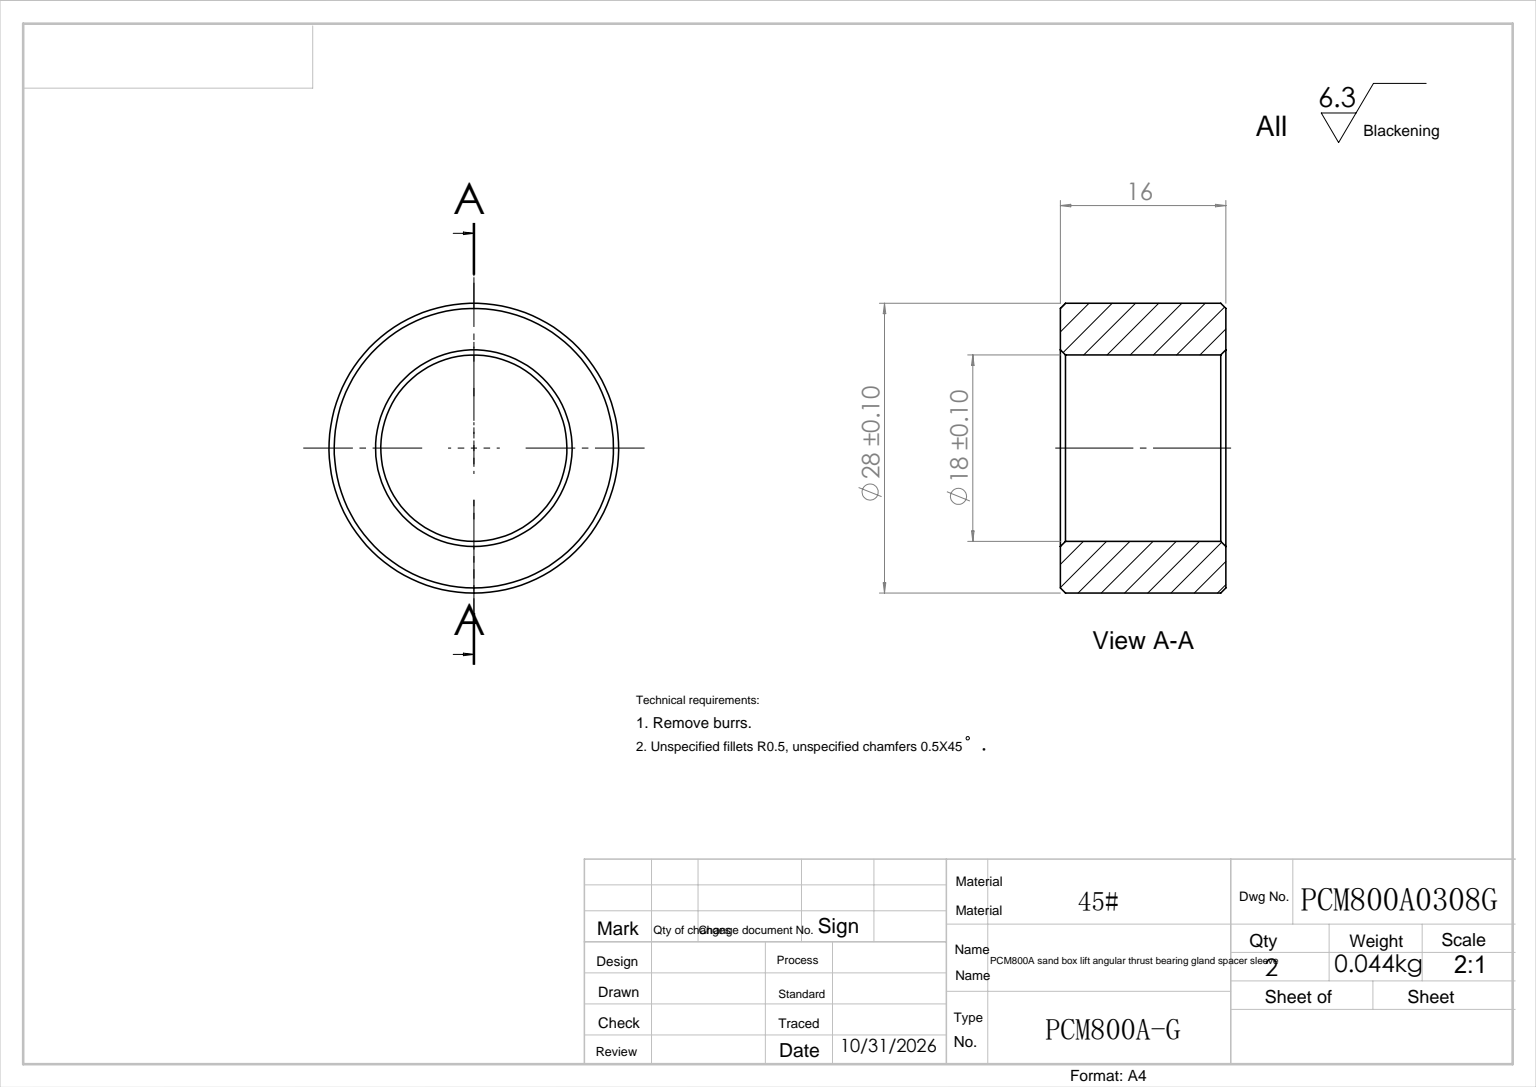
SolidWorks part; units mm, degrees
ref_plane "前视基准面" through (0, 0, 0) normal (0, 0, 1) x (1, 0, 0)
ref_plane "上视基准面" through (0, 0, 0) normal (0, 1, 0) x (1, 0, 0)
ref_plane "右视基准面" through (0, 0, 0) normal (1, 0, 0) x (0, 0, -1)
sketch "草图1" plane through (0, 0, 0) normal (0, 1, 0) x (1, 0, 0)
  circle A0 centre (0, 0) radius 14
  circle A1 centre (0, 0) radius 9
  dimension "D1" = 18
  dimension "D2" = 28
extrude "拉伸1" add sketch "草图1" along normal blind 16
chamfer "倒角1" distance 0.5 angle 45 4 edges at (0, 0, 9) (0, 0, 14) (0, 16, 14) (0, 16, 9)
